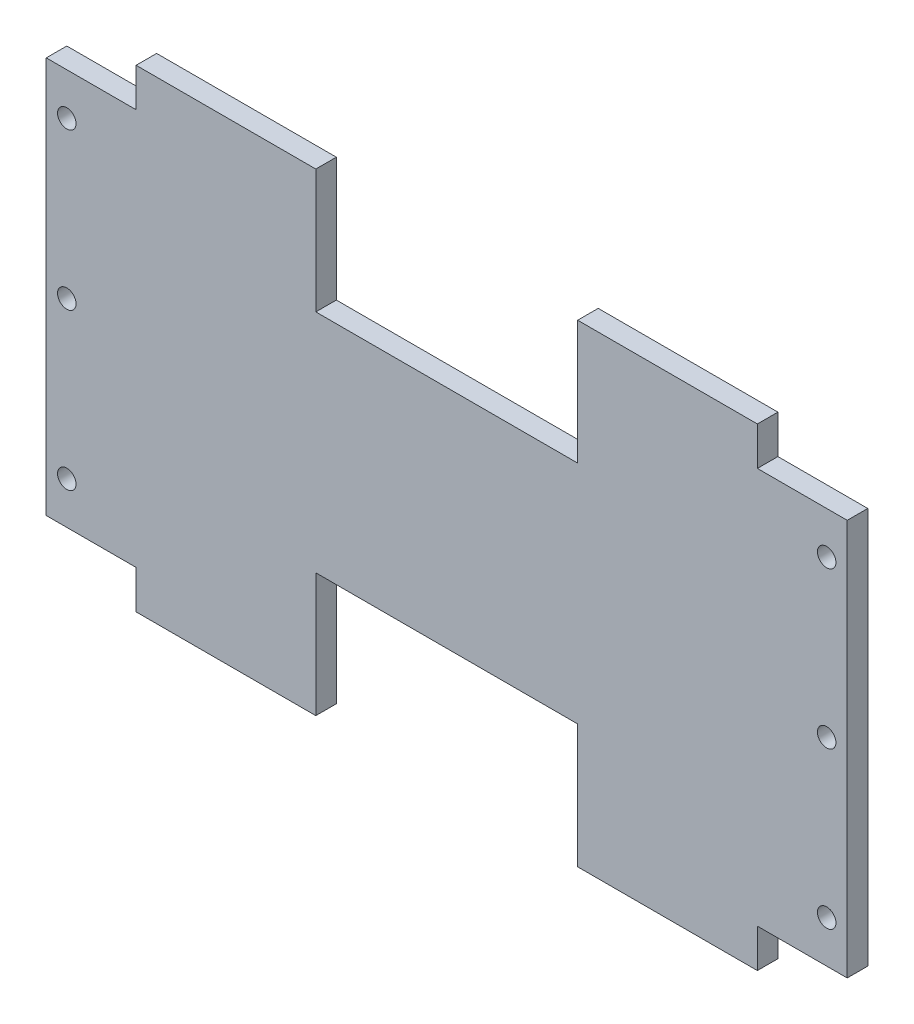
SolidWorks part; units mm, degrees
material "Q235"
ref_plane "Front Plane" through (0, 0, 0) normal (0, 0, 1) x (1, 0, 0)
ref_plane "Top Plane" through (0, 0, 0) normal (0, 1, 0) x (1, 0, 0)
ref_plane "Right Plane" through (0, 0, 0) normal (1, 0, 0) x (0, 0, -1)
sketch "Sketch1" plane through (0, 0, 0) normal (0, 0, 1) x (1, 0, 0)
  line L0 (255, 0) -> (-255, 0)
  line L1 (-255, 0) -> (-255, -241)
  line L2 (-255, -241) -> (-605, -241)
  line L3 (-605, -241) -> (-605, -166)
  line L4 (-605, -166) -> (-780, -166)
  line L5 (-780, -166) -> (-780, 606)
  line L6 (-780, 606) -> (-605, 606)
  line L7 (-605, 606) -> (-605, 681)
  line L8 (-605, 681) -> (-255, 681)
  line L9 (-255, 681) -> (-255, 440)
  line L10 (-255, 440) -> (255, 440)
  line L11 (0, 440) -> (0, 0) construction
  line L12 (255, 681) -> (255, 440)
  line L13 (605, 681) -> (255, 681)
  line L14 (605, 606) -> (605, 681)
  line L15 (780, 606) -> (605, 606)
  line L16 (780, -166) -> (780, 606)
  line L17 (605, -166) -> (780, -166)
  line L18 (605, -241) -> (605, -166)
  line L19 (255, -241) -> (605, -241)
  line L20 (255, 0) -> (255, -241)
  circle A0 centre (-740, 524) radius 18
  circle A1 centre (-740, 220) radius 18
  circle A2 centre (-740, -84) radius 18
  circle A3 centre (740, 220) radius 18
  circle A4 centre (740, 524) radius 18
  circle A5 centre (740, -84) radius 18
  dimension "D9" = 82
  dimension "D10" = 608
  dimension "D11" = 304
  dimension "D12" = 36
  dimension "D13" = 1480
  dimension "D1" = 1560
  dimension "D2" = 922
  dimension "D3" = 772
  dimension "D4" = 440
  dimension "D5" = 510
  dimension "D6" = 75
  dimension "D7" = 241
  dimension "D8" = 1210
extrude "Boss-Extrude1" add sketch "Sketch1" along normal blind 40
